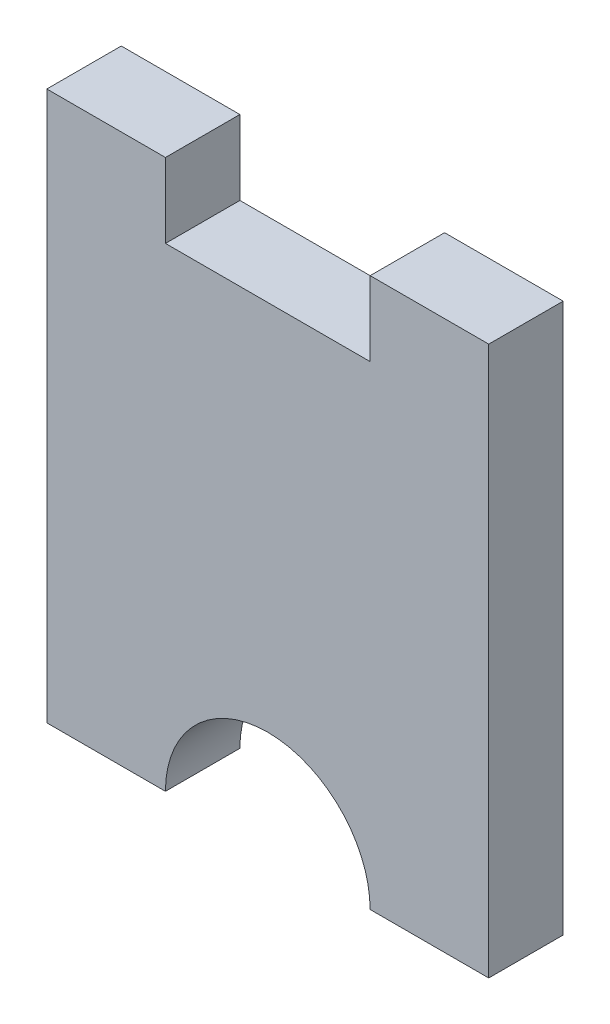
SolidWorks part; units mm, degrees
material "Q235B"
ref_plane "Front Plane" through (0, 0, 0) normal (0, 0, 1) x (1, 0, 0)
ref_plane "Top Plane" through (0, 0, 0) normal (0, 1, 0) x (1, 0, 0)
ref_plane "Right Plane" through (0, 0, 0) normal (1, 0, 0) x (0, 0, -1)
sketch "Sketch1" plane through (0, 0, 0) normal (0, 0, 1) x (1, 0, 0)
  line L0 (-194.5426, 40.1492) -> (-207.2903, 40.1492)
  line L1 (-194.5426, 40.1492) -> (-194.5426, 99.1492)
  line L2 (-194.5426, 99.1492) -> (-207.288, 99.1492)
  line L3 (-207.288, 99.1492) -> (-207.288, 91.1492)
  line L4 (-218.2903, 40.1492) -> (-218.288, 93.9497) construction
  line L5 (-242.038, 99.1492) -> (-242.038, 40.1492)
  line L6 (-242.038, 40.1492) -> (-229.2903, 40.1492)
  line L7 (-242.038, 40.1492) -> (-242.038, 101.3418) construction
  line L8 (-229.288, 91.1492) -> (-207.288, 91.1492)
  line L9 (-229.288, 99.1492) -> (-229.288, 91.1492)
  line L10 (-242.038, 99.1492) -> (-229.288, 99.1492)
  arc A0 (-207.2903, 40.1492) -> (-229.2903, 40.1492) centre (-218.2903, 40.1492) ccw
  dimension "D4" = 11
  dimension "D1" = 12.7477
  dimension "D2" = 12.7477
  dimension "D3" = 47.4955
  dimension "D5" = 23.7477
  dimension "D6" = 8
  dimension "D7" = 90
  dimension "D8" = 12.75
  dimension "D9" = 90
  dimension "D10" = 59
  dimension "D11" = 22
  dimension "D12" = 59
extrude "Boss-Extrude1" add sketch "Sketch1" along normal blind 8
